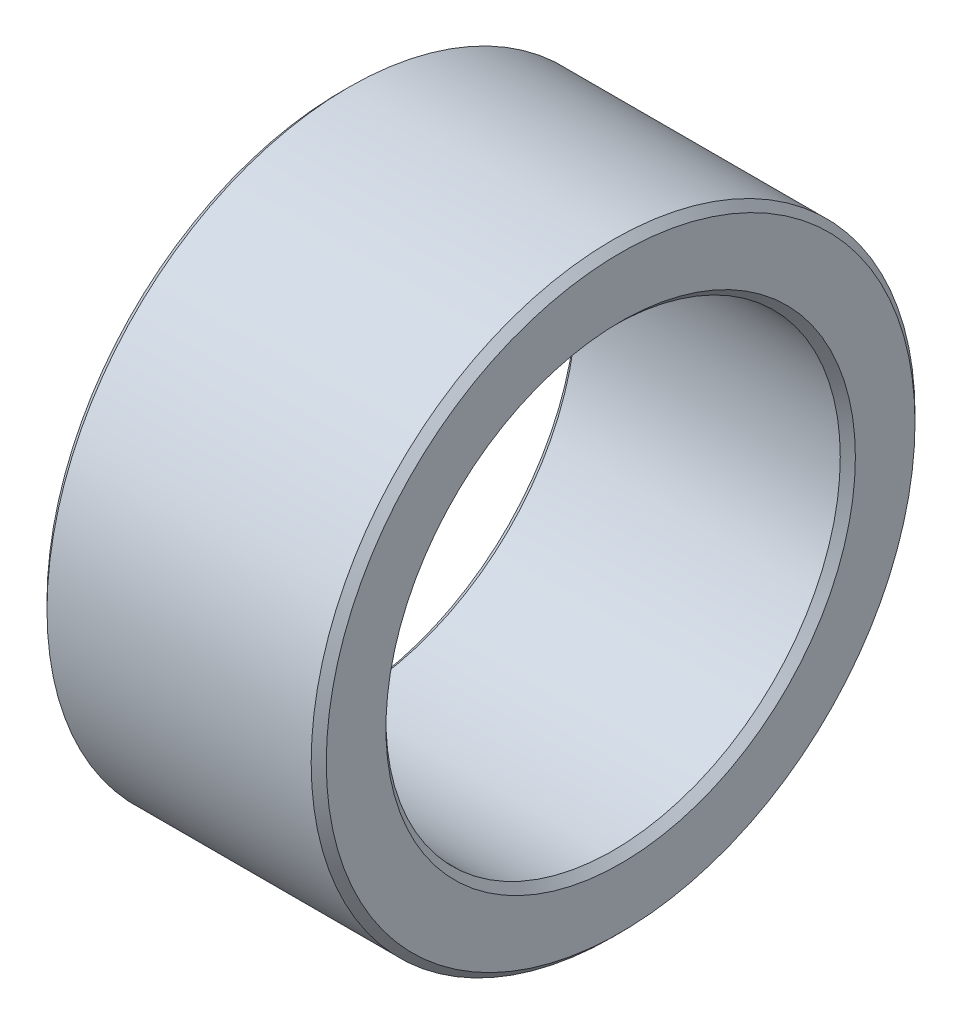
from build123d import *

# Parameters (mm, degrees)
SKETCH_1_R      = 20
SKETCH_1_R_2    = 15.05
EXTRUDE_1_DEPTH = 18.5
CHAMFER_1_SIZE  = 0.5


with BuildPart() as part:
    # 草图1 → 凸台-拉伸1 (new body)
    with BuildSketch(Plane(origin=(0, 0, 0), x_dir=(0, 0, -1), z_dir=(1, 0, 0))):
        Circle(SKETCH_1_R)
        Circle(SKETCH_1_R_2, mode=Mode.SUBTRACT)
    extrude(amount=EXTRUDE_1_DEPTH)

    # 倒角1
    chamfer_1_edges = [part.edges().sort_by_distance(p)[0] for p in [
        (0, 0, 20),
        (18.5, 0, 20),
        (0, 0, 15.05),
        (18.5, 0, 15.05),
    ]]
    chamfer(chamfer_1_edges, length=CHAMFER_1_SIZE)


solid = part.part
